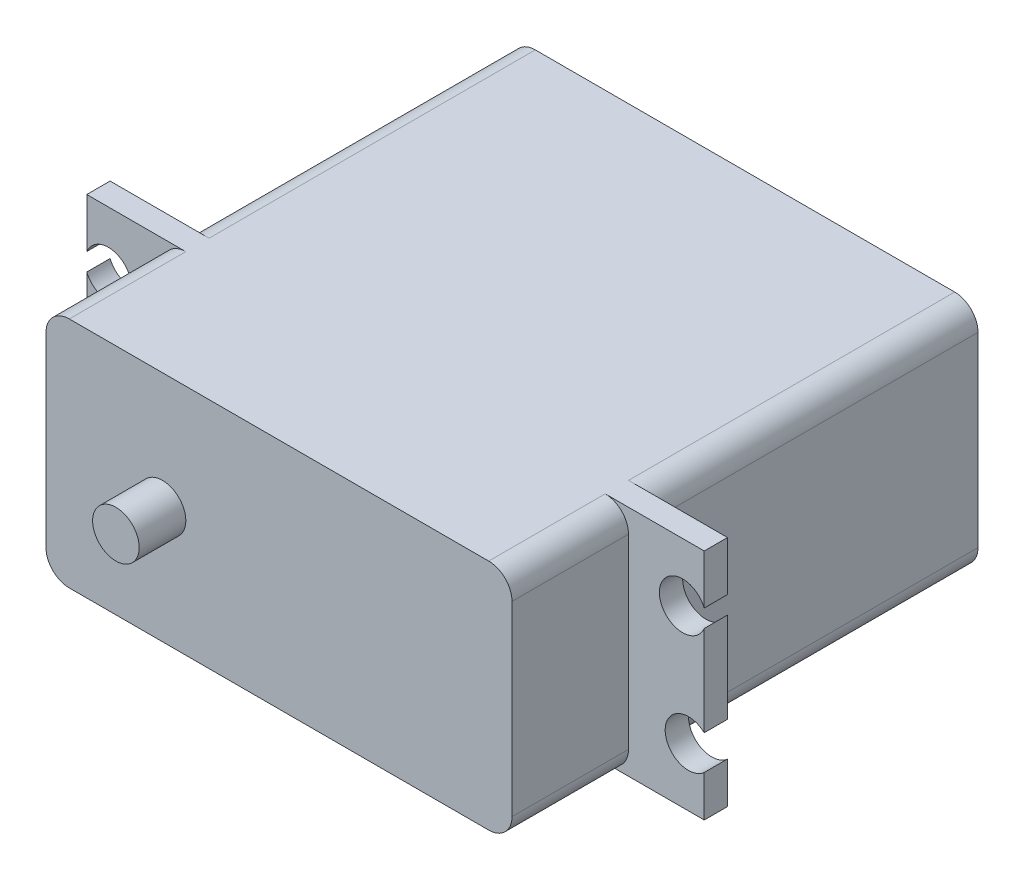
from build123d import *

# Parameters (mm, degrees)
SKETCH1_W           = 40
SKETCH1_H           = 40
BOSS_EXTRUDE1_DEPTH = 20
SKETCH2_W           = 6.5
SKETCH2_H           = 20
BOSS_EXTRUDE2_DEPTH = 2
SKETCH3_R           = 2
CUT_EXTRUDE1_DEPTH  = 2
SKETCH4_R           = 2
BOSS_EXTRUDE3_DEPTH = 4
FILLET1_R           = 2


with BuildPart() as part:
    # Sketch1 → Boss-Extrude1 (new body)
    with BuildSketch(Plane(origin=(0, 0, 0), x_dir=(1, 0, 0), z_dir=(0, 1, 0))):
        Rectangle(SKETCH1_W, SKETCH1_H)
    extrude(amount=BOSS_EXTRUDE1_DEPTH)

    # Sketch2 → Boss-Extrude2 (add)
    with BuildSketch(Plane(origin=(0, 0, 8), x_dir=(-1, 0, 0), z_dir=(0, 0, -1))):
        with Locations((23.25, 10)):
            Rectangle(SKETCH2_W, SKETCH2_H)
        with Locations((-23.25, 10)):
            Rectangle(SKETCH2_W, SKETCH2_H)
    extrude(amount=-BOSS_EXTRUDE2_DEPTH)

    # Sketch3 → Cut-Extrude1 (cut)
    with BuildSketch(Plane(origin=(0, 0, 8), x_dir=(-1, 0, 0), z_dir=(0, 0, -1))):
        with Locations((25.149376169, 5.012476611)):
            Circle(SKETCH3_R)
        with Locations((24.65, 15)):
            Circle(SKETCH3_R)
    cut_extrude1 = extrude(amount=-CUT_EXTRUDE1_DEPTH, mode=Mode.SUBTRACT)

    # Mirror2: Cut-Extrude1 across plane
    add(cut_extrude1.mirror(Plane.ZY), mode=Mode.SUBTRACT)

    # Sketch4 → Boss-Extrude3 (add)
    with BuildSketch(Plane.XY.offset(20)):
        with Locations(Location((-10, 10, 0), (0, 0, 180))):
            Circle(SKETCH4_R)
    extrude(amount=BOSS_EXTRUDE3_DEPTH)

    # Fillet1
    fillet1_edges = [part.edges().sort_by_distance(p)[0] for p in [
        (20, 20, -6),
        (20, 20, 15),
        (20, 0, -6),
        (20, 0, 15),
        (-20, 0, 15),
        (-20, 0, -6),
        (-20, 20, 15),
        (-20, 20, -6),
    ]]
    fillet(fillet1_edges, radius=FILLET1_R)


solid = part.part
